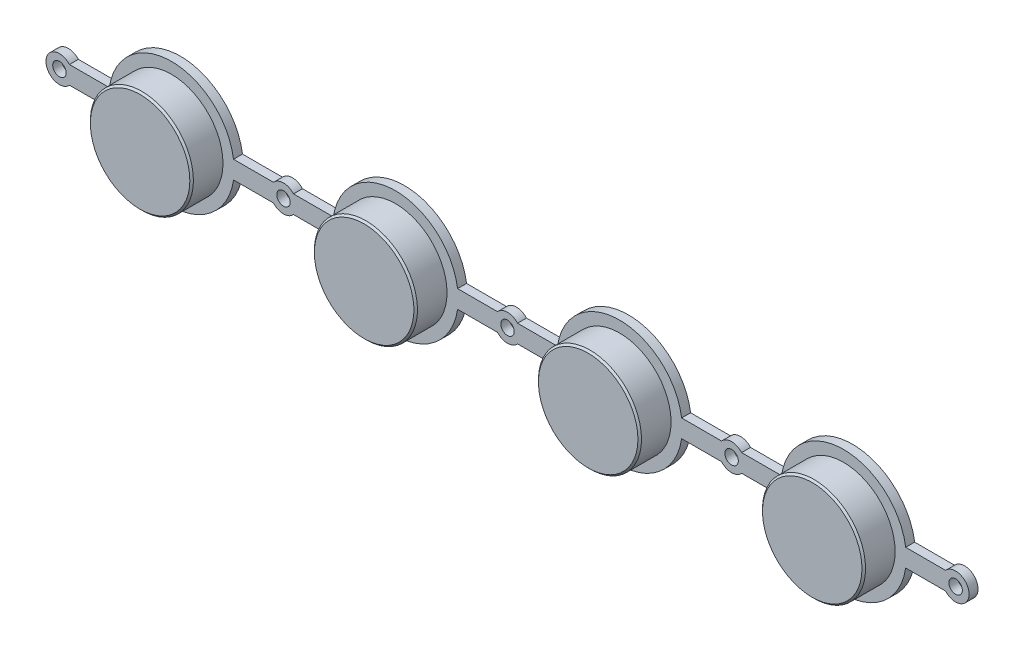
from build123d import *

# Parameters (mm, degrees)
SKETCH1_R           = 0.75
BOSS_EXTRUDE1_DEPTH = 1
SKETCH2_R           = 5.75
BOSS_EXTRUDE2_DEPTH = 3.5
CHAMFER1_SIZE       = 0.2
BOSS_EXTRUDE3_DEPTH = 2
CHAMFER2_SIZE       = 1.6


with BuildPart() as part:
    # Sketch1 → Boss-Extrude1 (new body)
    with BuildSketch(Plane.XY):
        with BuildLine():
            Line((-11.381966011, 1), (-6.92820323, 1))
            ThreePointArc((-6.92820323, 1), (0, 7), (6.92820323, 1))
            Line((6.92820323, 1), (11.381966011, 1))
            ThreePointArc((11.381966011, 1), (12.5, 1.5), (13.618033989, 1))
            Line((13.618033989, 1), (18.07179677, 1))
            ThreePointArc((18.07179677, 1), (25, 7), (31.92820323, 1))
            Line((31.92820323, 1), (36.381966011, 1))
            ThreePointArc((36.381966011, 1), (37.5, 1.5), (38.618033989, 1))
            Line((38.618033989, 1), (43.07179677, 1))
            ThreePointArc((43.07179677, 1), (50, 7), (56.92820323, 1))
            Line((56.92820323, 1), (61.381966011, 1))
            ThreePointArc((61.381966011, 1), (62.5, 1.5), (63.618033989, 1))
            Line((63.618033989, 1), (68.07179677, 1))
            ThreePointArc((68.07179677, 1), (75, 7), (81.92820323, 1))
            Line((81.92820323, 1), (86.381966011, 1))
            ThreePointArc((86.381966011, 1), (89, 0), (86.381966011, -1))
            Line((86.381966011, -1), (81.92820323, -1))
            ThreePointArc((81.92820323, -1), (75, -7), (68.07179677, -1))
            Line((68.07179677, -1), (63.618033989, -1))
            ThreePointArc((63.618033989, -1), (62.5, -1.5), (61.381966011, -1))
            Line((61.381966011, -1), (56.92820323, -1))
            ThreePointArc((56.92820323, -1), (50, -7), (43.07179677, -1))
            Line((43.07179677, -1), (38.618033989, -1))
            ThreePointArc((38.618033989, -1), (37.5, -1.5), (36.381966011, -1))
            Line((36.381966011, -1), (31.92820323, -1))
            ThreePointArc((31.92820323, -1), (25, -7), (18.07179677, -1))
            Line((18.07179677, -1), (13.618033989, -1))
            ThreePointArc((13.618033989, -1), (12.5, -1.5), (11.381966011, -1))
            Line((11.381966011, -1), (6.92820323, -1))
            ThreePointArc((6.92820323, -1), (0, -7), (-6.92820323, -1))
            Line((-6.92820323, -1), (-11.381966011, -1))
            ThreePointArc((-11.381966011, -1), (-14, 0), (-11.381966011, 1))
        make_face()
        with Locations((12.5, 0)):
            Circle(SKETCH1_R, mode=Mode.SUBTRACT)
        with Locations((37.5, 0)):
            Circle(SKETCH1_R, mode=Mode.SUBTRACT)
        with Locations((62.5, 0)):
            Circle(SKETCH1_R, mode=Mode.SUBTRACT)
        with Locations((-12.5, 0)):
            Circle(SKETCH1_R, mode=Mode.SUBTRACT)
        with Locations((87.5, 0)):
            Circle(SKETCH1_R, mode=Mode.SUBTRACT)
    extrude(amount=BOSS_EXTRUDE1_DEPTH)

    # Sketch2 → Boss-Extrude2 (add)
    with BuildSketch(Plane.XY.offset(1)):
        Circle(SKETCH2_R)
        with Locations((25, 0)):
            Circle(SKETCH2_R)
        with Locations((50, 0)):
            Circle(SKETCH2_R)
        with Locations((75, 0)):
            Circle(SKETCH2_R)
    extrude(amount=BOSS_EXTRUDE2_DEPTH)

    # Chamfer1
    chamfer1_edges = [part.edges().sort_by_distance(p)[0] for p in [
        (-5.75, 0, 4.5),
        (19.25, 0, 4.5),
        (44.25, 0, 4.5),
        (69.25, 0, 4.5),
    ]]
    chamfer(chamfer1_edges, length=CHAMFER1_SIZE)

    # Sketch3 → Boss-Extrude3 (add)
    with BuildSketch(Plane(origin=(0, 0, 0), x_dir=(-1, 0, 0), z_dir=(0, 0, -1))):
        Polygon((-74.25, -0.75), (-74.25, -4), (-75.75, -4), (-75.75, -0.75), (-79, -0.75), (-79, 0.75), (-75.75, 0.75), (-75.75, 4), (-74.25, 4), (-74.25, 0.75), (-71, 0.75), (-71, -0.75), align=None)
        Polygon((-50.75, 4), (-49.25, 4), (-49.25, 0.75), (-46, 0.75), (-46, -0.75), (-49.25, -0.75), (-49.25, -4), (-50.75, -4), (-50.75, -0.75), (-54, -0.75), (-54, 0.75), (-50.75, 0.75), align=None)
        Polygon((-29, 0.75), (-25.75, 0.75), (-25.75, 4), (-24.25, 4), (-24.25, 0.75), (-21, 0.75), (-21, -0.75), (-24.25, -0.75), (-24.25, -4), (-25.75, -4), (-25.75, -0.75), (-29, -0.75), align=None)
        Polygon((-4, 0.75), (-0.75, 0.75), (-0.75, 4), (0.75, 4), (0.75, 0.75), (4, 0.75), (4, -0.75), (0.75, -0.75), (0.75, -4), (-0.75, -4), (-0.75, -0.75), (-4, -0.75), align=None)
    extrude(amount=BOSS_EXTRUDE3_DEPTH)

    # Chamfer2
    chamfer2_edges = [part.edges().sort_by_distance(p)[0] for p in [
        (75, -4, -2),
        (71, 0, -2),
        (75, 4, -2),
        (79, 0, -2),
        (46, 0, -2),
        (50, 4, -2),
        (54, 0, -2),
        (50, -4, -2),
        (21, 0, -2),
        (25, 4, -2),
        (29, 0, -2),
        (25, -4, -2),
        (-4, 0, -2),
        (0, 4, -2),
        (4, 0, -2),
        (0, -4, -2),
    ]]
    chamfer(chamfer2_edges, length=CHAMFER2_SIZE)


solid = part.part
